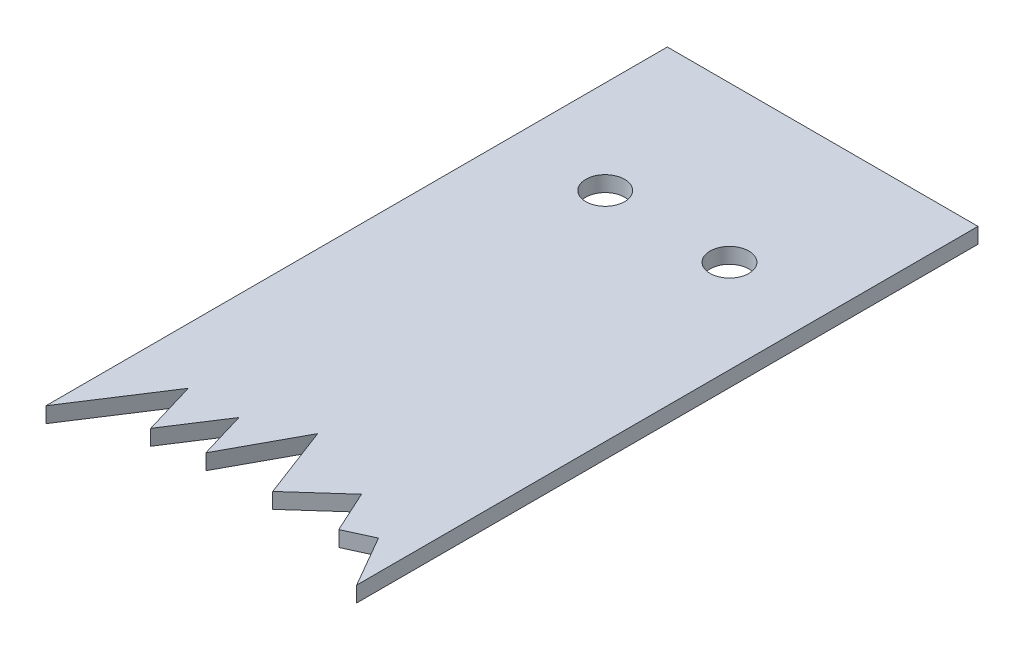
SolidWorks part; units mm, degrees
ref_plane "Front Plane" through (0, 0, 0) normal (0, 0, 1) x (1, 0, 0)
ref_plane "Top Plane" through (0, 0, 0) normal (0, 1, 0) x (1, 0, 0)
ref_plane "Right Plane" through (0, 0, 0) normal (1, 0, 0) x (0, 0, -1)
sketch "Sketch1" plane through (0, 0, 0) normal (0, 1, 0) x (1, 0, 0)
  line L1 (-20, 40) -> (20, 40)
  line L2 (-20, 40) -> (-20, -40)
  line L3 (-20, -40) -> (20, -40)
  line L4 (20, 40) -> (20, -40)
  line L5 (-20, 40) -> (20, -40) construction
  line L6 (-20, -40) -> (20, 40) construction
  point P0 (0, 0)
  dimension "D1" = 40
  dimension "D2" = 80
extrude "Boss-Extrude1" add sketch "Sketch1" along normal blind 2
sketch "Sketch2" plane through (0, 0, 0) normal (0, -1, 0) x (1, 0, 0)
  circle A0 centre (8, -20) radius 2.5
  circle A1 centre (-8, -20) radius 2.5
  dimension "D1" = 5
extrude "Cut-Extrude1" cut sketch "Sketch2" against normal blind 10
sketch "Sketch3" plane through (0, 2, 0) normal (0, 1, 0) x (1, 0, 0)
  line L0 (-20, -40) -> (-12.7846, -28.8913)
  line L1 (-12.7846, -28.8913) -> (-10.737, -35.7787)
  line L2 (-10.737, -35.7787) -> (-6.2635, -28.8913)
  line L3 (-6.2635, -28.8913) -> (-4.4594, -34.9597)
  line L4 (-4.4594, -34.9597) -> (0.6034, -25.613)
  line L5 (0.6034, -25.613) -> (4.1546, -34.9597)
  line L6 (4.1546, -34.9597) -> (10.1809, -29.5599)
  line L7 (10.1809, -29.5599) -> (12.6553, -34.9597)
  line L8 (12.6553, -34.9597) -> (16.1611, -33.3532)
  line L9 (16.1611, -33.3532) -> (20, -40)
  line L10 (20, -40) -> (-20, -40)
extrude "Cut-Extrude2" cut sketch "Sketch3" against normal blind 10
